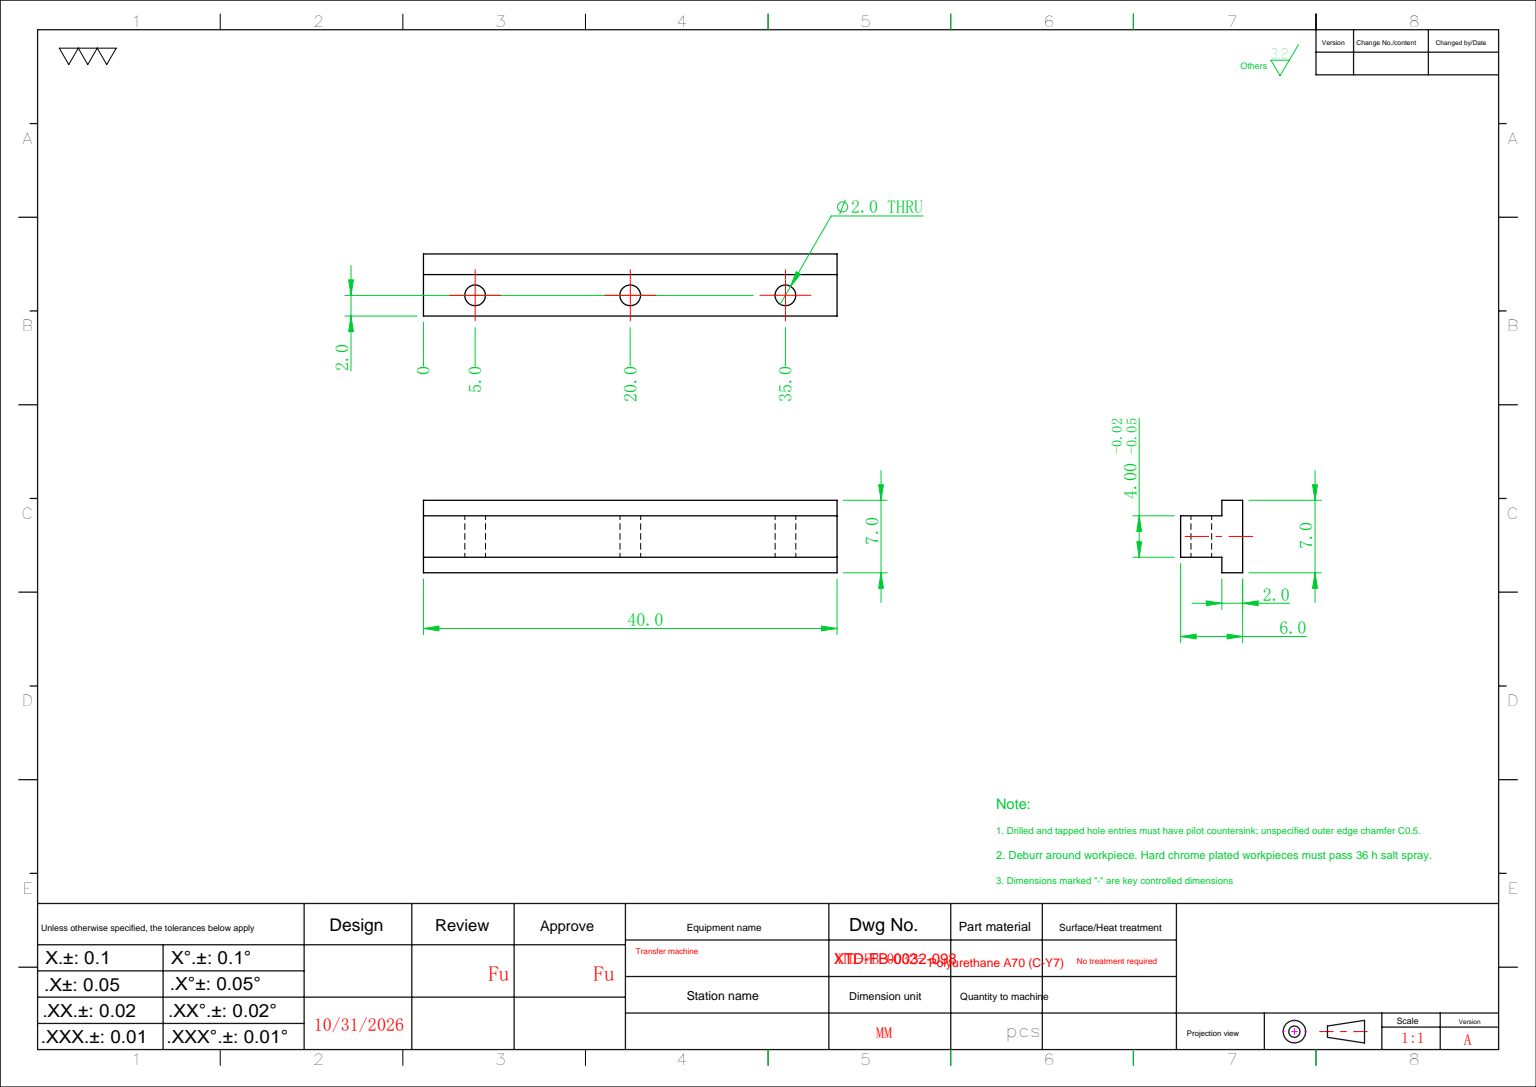
from build123d import *

# Parameters (mm, degrees)
SKETCH_1_W          = 40
SKETCH_1_H          = 4
EXTRUDE_1_DEPTH     = 4
SKETCH_2_W          = 2
SKETCH_2_H          = 7
EXTRUDE_2_DEPTH     = 40
SKETCH_3_R          = 1
CUT_EXTRUDE_1_DEPTH = 22.124630174


with BuildPart() as part:
    # 草图1 → 凸台-拉伸1 (new body)
    with BuildSketch(Plane.XY):
        Rectangle(SKETCH_1_W, SKETCH_1_H)
    extrude(amount=EXTRUDE_1_DEPTH)

    # 草图2 → 凸台-拉伸2 (add)
    with BuildSketch(Plane(origin=(20, 0, 0), x_dir=(0, 0, -1), z_dir=(1, 0, 0))):
        with Locations((1, 0)):
            Rectangle(SKETCH_2_W, SKETCH_2_H)
    extrude(amount=-EXTRUDE_2_DEPTH)

    # 草图3 → 切除-拉伸1 (cut, through all)
    with BuildSketch(Plane(origin=(0, 2, 0), x_dir=(1, 0, 0), z_dir=(0, 1, 0))):
        with Locations(Location((-15, -2, 0), (0, 0, 270))):
            Circle(SKETCH_3_R)
        with Locations(Location((0, -2, 0), (0, 0, 270))):
            Circle(SKETCH_3_R)
        with Locations(Location((15, -2, 0), (0, 0, 270))):
            Circle(SKETCH_3_R)
    extrude(amount=-CUT_EXTRUDE_1_DEPTH, mode=Mode.SUBTRACT)


solid = part.part
